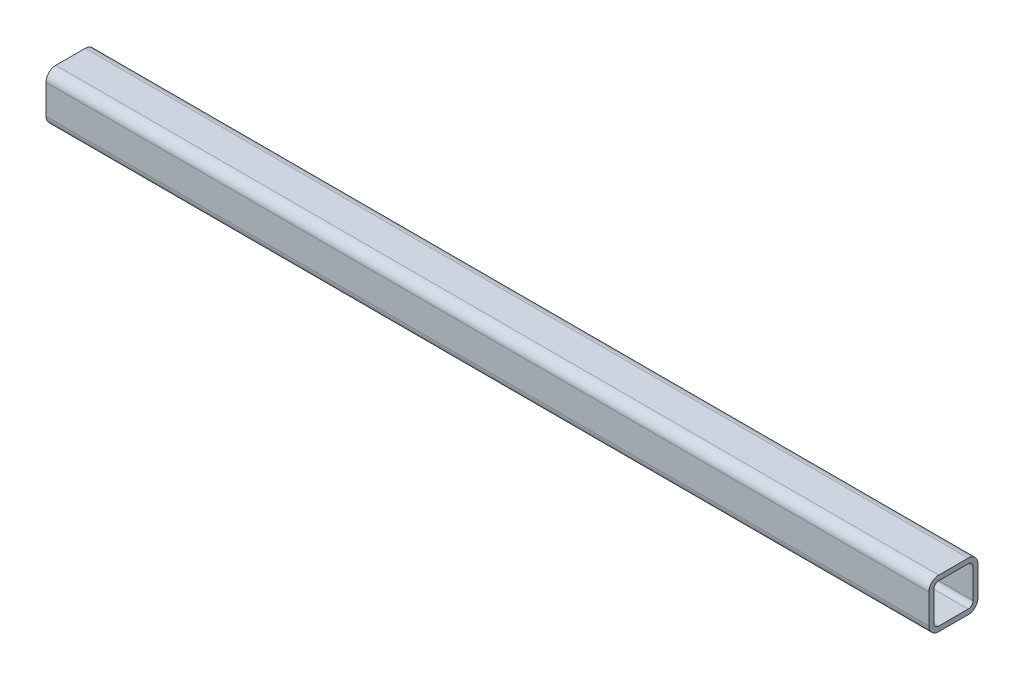
from build123d import *

# Parameters (mm, degrees)
SQUARE_TUBE_40_X_40_X_4_1_DEPTH = 720


with BuildPart() as part:
    # Sketch1 → Square Tube 40 X 40 X 4(1) (new body)
    with BuildSketch(Plane.YZ.offset(-1000)):
        with BuildLine():
            Line((-12, -20), (12, -20))
            ThreePointArc((12, -20), (17.656854249, -17.656854249), (20, -12))
            Line((20, -12), (20, 12))
            ThreePointArc((20, 12), (17.656854249, 17.656854249), (12, 20))
            Line((12, 20), (-12, 20))
            ThreePointArc((-12, 20), (-17.656854249, 17.656854249), (-20, 12))
            Line((-20, 12), (-20, -12))
            ThreePointArc((-20, -12), (-17.656854249, -17.656854249), (-12, -20))
        make_face()
        with BuildLine():
            Line((-12, -16), (12, -16))
            ThreePointArc((12, -16), (14.828427125, -14.828427125), (16, -12))
            Line((16, -12), (16, 12))
            ThreePointArc((16, 12), (14.828427125, 14.828427125), (12, 16))
            Line((12, 16), (-12, 16))
            ThreePointArc((-12, 16), (-14.828427125, 14.828427125), (-16, 12))
            Line((-16, 12), (-16, -12))
            ThreePointArc((-16, -12), (-14.828427125, -14.828427125), (-12, -16))
        make_face(mode=Mode.SUBTRACT)
    extrude(amount=SQUARE_TUBE_40_X_40_X_4_1_DEPTH)


solid = part.part
